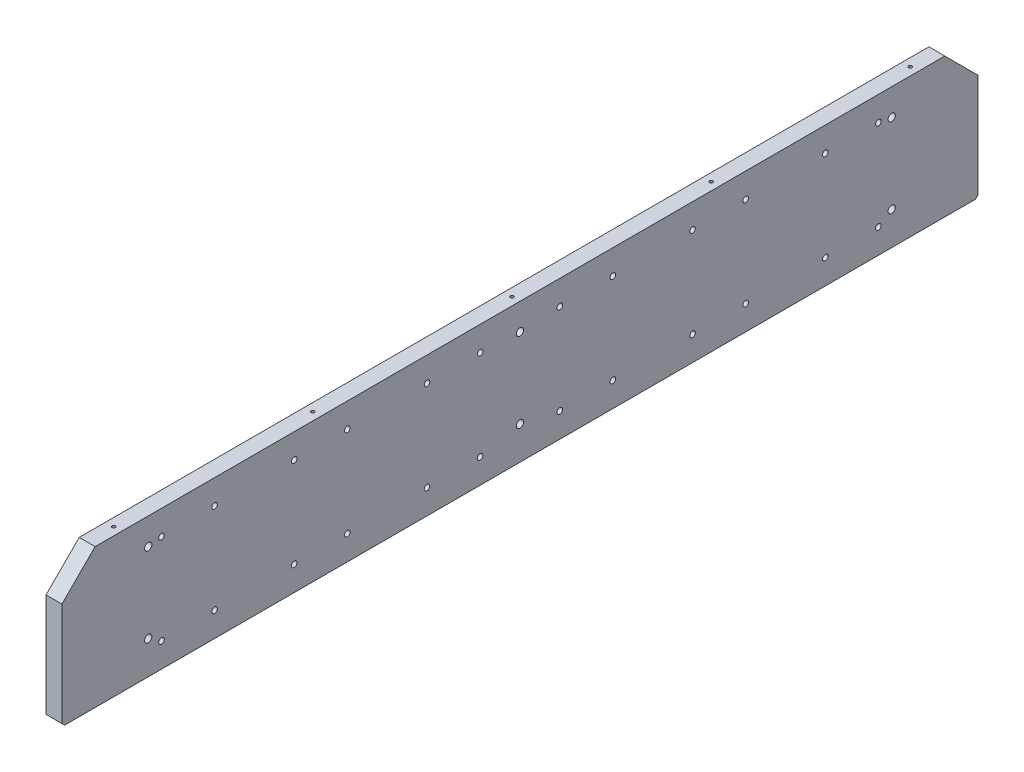
SolidWorks part; units mm, degrees
material "A6061"
ref_plane "前基準面" through (0, 0, 0) normal (0, 0, 1) x (1, 0, 0)
ref_plane "上基準面" through (0, 0, 0) normal (0, 1, 0) x (1, 0, 0)
ref_plane "右基準面" through (0, 0, 0) normal (1, 0, 0) x (0, 0, -1)
sketch "草图1" plane through (0, 0, 0) normal (1, 0, 0) x (0, 0, -1)
  line L1 (-345, 52.5) -> (345, 52.5)
  line L2 (-345, 52.5) -> (-345, -52.5)
  line L3 (-345, -52.5) -> (345, -52.5)
  line L4 (345, 52.5) -> (345, -52.5)
  line L5 (-345, 52.5) -> (345, -52.5) construction
  line L6 (-345, -52.5) -> (345, 52.5) construction
  point P0 (0, 0)
  dimension "D1" = 105
  dimension "D2" = 690
extrude "凸台-拉伸1" add sketch "草图1" along normal mid plane 12
chamfer "倒角1" distance 2 angle 45 2 edges at (0, -52.5, -345) (0, -52.5, 345)
chamfer "倒角2" distance 25 angle 45 2 edges at (0, 52.5, 345) (0, 52.5, -345)
hole_wizard "M6 螺纹孔1" positions "草图4" profile "草图5" tap size "M6" standard "GB"
sketch "草图4" plane through (0, -52.5, 0) normal (0, -1, 0) x (-1, 0, 0)
  point P0 (0, -300)
  point P5 (0, -150)
  point P6 (0, 0)
  point P7 (0, 150)
  point P8 (0, 300)
  dimension "D2" = 150
  dimension "D1" = 5
sketch "草图5" plane through (0, -52.5, 300) normal (1, 0, 0) x (0, 0, -1)
  line L0 (0, 0) -> (0, 16.5022)
  line L1 (0, 16.5022) -> (2.5, 15)
  line L2 (2.5, 15) -> (2.5, 0)
  line L5 (2.5, 0) -> (0, 0)
  line L10 (0, 16.5022) -> (-2.5, 15) construction
  line L11 (0, -6.35) -> (0, 107.95) construction
  dimension "螺纹孔钻头直径" = 5
  dimension "螺纹孔钻头深度" = 15
  dimension "导头角度" = 118
cosmetic thread "孔螺蚊线2" parameters "D1"=12, "D2"=6
cosmetic thread "孔螺蚊线3" parameters "D1"=12, "D2"=6
cosmetic thread "孔螺蚊线4" parameters "D1"=12, "D2"=6
cosmetic thread "孔螺蚊线51" parameters "D1"=12, "D2"=6
cosmetic thread "孔螺蚊线52" parameters "D1"=12, "D2"=6
hole_wizard "打孔尺寸(%根据)内六角圆柱头螺钉的类型1" positions "草图6" profile "草图7" counterbore size "M5" standard "GB" end condition through all
sketch "草图6" plane through (-6, 0, 0) normal (-1, 0, 0) x (0, 0, 1)
  line L0 (343, -52.5) -> (-343, -52.5) construction
  point P0 (280, 32.5)
  point P2 (280, -27.5)
  point P6 (0, 32.5)
  point P7 (0, -27.5)
  point P8 (-280, 32.5)
  point P9 (-280, -27.5)
  dimension "D2" = 280
  dimension "D3" = 25
  dimension "D4" = 60
  dimension "D1" = 3
sketch "草图7" plane through (-6, 32.5, 280) normal (0, 1, 0) x (0, 0, 1)
  line L0 (0, 0) -> (0, 12)
  line L1 (0, 12) -> (2.75, 12)
  line L3 (2.75, 12) -> (2.75, 5.7)
  line L4 (2.75, 5.7) -> (5, 5.7)
  line L5 (5, 5.7) -> (5, 0)
  line L7 (5, 0) -> (0, 0)
  line L11 (0, -6.35) -> (0, 107.95) construction
  dimension "通孔孔直径" = 5.5
  dimension "通孔孔深度" = 12
  dimension "柱形沉头孔直径" = 10
  dimension "柱形沉头孔深度" = 5.7
hole_wizard "M5 螺纹孔1" positions "草图8" profile "草图9" tap size "M5" standard "GB" end condition through all
sketch "草图8" plane through (-6, 0, 0) normal (-1, 0, 0) x (0, 0, 1)
  line L0 (345, 27.5) -> (345, -50.5) construction
  line L1 (-320, 52.5) -> (320, 52.5) construction
  line L2 (0, 0) -> (0, -134.9884) construction
  point P0 (270, 34)
  point P2 (270, -34)
  point P8 (170, 34)
  point P9 (170, -34)
  point P10 (70, 34)
  point P11 (70, -34)
  point P12 (-30, 34)
  point P13 (-30, -34)
  point P14 (-130, 34)
  point P15 (-130, -34)
  point P39 (130, -34)
  point P40 (130, 34)
  point P41 (30, -34)
  point P42 (30, 34)
  point P43 (-70, -34)
  point P44 (-70, 34)
  point P45 (-170, -34)
  point P46 (-170, 34)
  point P47 (-270, -34)
  point P48 (-270, 34)
  point P52 (-230, 34)
  point P53 (-230, -34)
  point P57 (230, -34)
  point P58 (230, 34)
  dimension "D1" = 6
  dimension "D2" = 68
  dimension "D3" = 75
  dimension "D4" = 18.5
  dimension "D5" = 100
sketch "草图9" plane through (-6, 34, 270) normal (0, 1, 0) x (0, 0, 1)
  line L0 (0, 0) -> (0, 12)
  line L1 (0, 12) -> (2.1, 12)
  line L2 (2.1, 12) -> (2.1, 0)
  line L5 (2.1, 0) -> (0, 0)
  line L11 (0, -6.35) -> (0, 107.95) construction
  dimension "通孔螺纹孔钻头直径" = 4.2
  dimension "通孔螺纹孔钻头深度" = 12
cosmetic thread "孔螺蚊线7" parameters "D2"=5
cosmetic thread "孔螺蚊线8" parameters "D2"=5
cosmetic thread "孔螺蚊线16" parameters "D2"=5
cosmetic thread "孔螺蚊线17" parameters "D2"=5
cosmetic thread "孔螺蚊线25" parameters "D2"=5
cosmetic thread "孔螺蚊线26" parameters "D2"=5
cosmetic thread "孔螺蚊线27" parameters "D2"=5
cosmetic thread "孔螺蚊线28" parameters "D2"=5
cosmetic thread "孔螺蚊线29" parameters "D2"=5
cosmetic thread "孔螺蚊线30" parameters "D2"=5
cosmetic thread "孔螺蚊线33" parameters "D2"=5
cosmetic thread "孔螺蚊线34" parameters "D2"=5
cosmetic thread "孔螺蚊线53" parameters "D2"=5
cosmetic thread "孔螺蚊线54" parameters "D2"=5
cosmetic thread "孔螺蚊线55" parameters "D2"=5
cosmetic thread "孔螺蚊线56" parameters "D2"=5
cosmetic thread "孔螺蚊线57" parameters "D2"=5
cosmetic thread "孔螺蚊线58" parameters "D2"=5
cosmetic thread "孔螺蚊线59" parameters "D2"=5
cosmetic thread "孔螺蚊线60" parameters "D2"=5
cosmetic thread "孔螺蚊线61" parameters "D2"=5
cosmetic thread "孔螺蚊线62" parameters "D2"=5
cosmetic thread "孔螺蚊线63" parameters "D2"=5
cosmetic thread "孔螺蚊线64" parameters "D2"=5
hole_wizard "M3 螺纹孔2" positions "草图12" profile "草图13" tap size "M3" standard "GB"
sketch "草图12" plane through (0, 52.5, 0) normal (0, 1, 0) x (1, 0, 0)
  point P0 (0, -300)
  point P6 (0, -150)
  point P7 (0, 0)
  point P8 (0, 150)
  point P9 (0, 300)
  dimension "D2" = 150
  dimension "D1" = 5
sketch "草图13" plane through (0, 52.5, 300) normal (1, 0, 0) x (0, 0, 1)
  line L0 (0, 0) -> (0, 8.2511)
  line L1 (0, 8.2511) -> (1.25, 7.5)
  line L2 (1.25, 7.5) -> (1.25, 0)
  line L5 (1.25, 0) -> (0, 0)
  line L10 (0, 8.2511) -> (-1.25, 7.5) construction
  line L11 (0, -6.35) -> (0, 107.95) construction
  dimension "螺纹孔钻头直径" = 2.5
  dimension "螺纹孔钻头深度" = 7.5
  dimension "导头角度" = 118
cosmetic thread "孔螺蚊线46" parameters "D1"=6, "D2"=3
cosmetic thread "孔螺蚊线47" parameters "D1"=6, "D2"=3
cosmetic thread "孔螺蚊线48" parameters "D1"=6, "D2"=3
cosmetic thread "孔螺蚊线49" parameters "D1"=6, "D2"=3
cosmetic thread "孔螺蚊线50" parameters "D1"=6, "D2"=3
